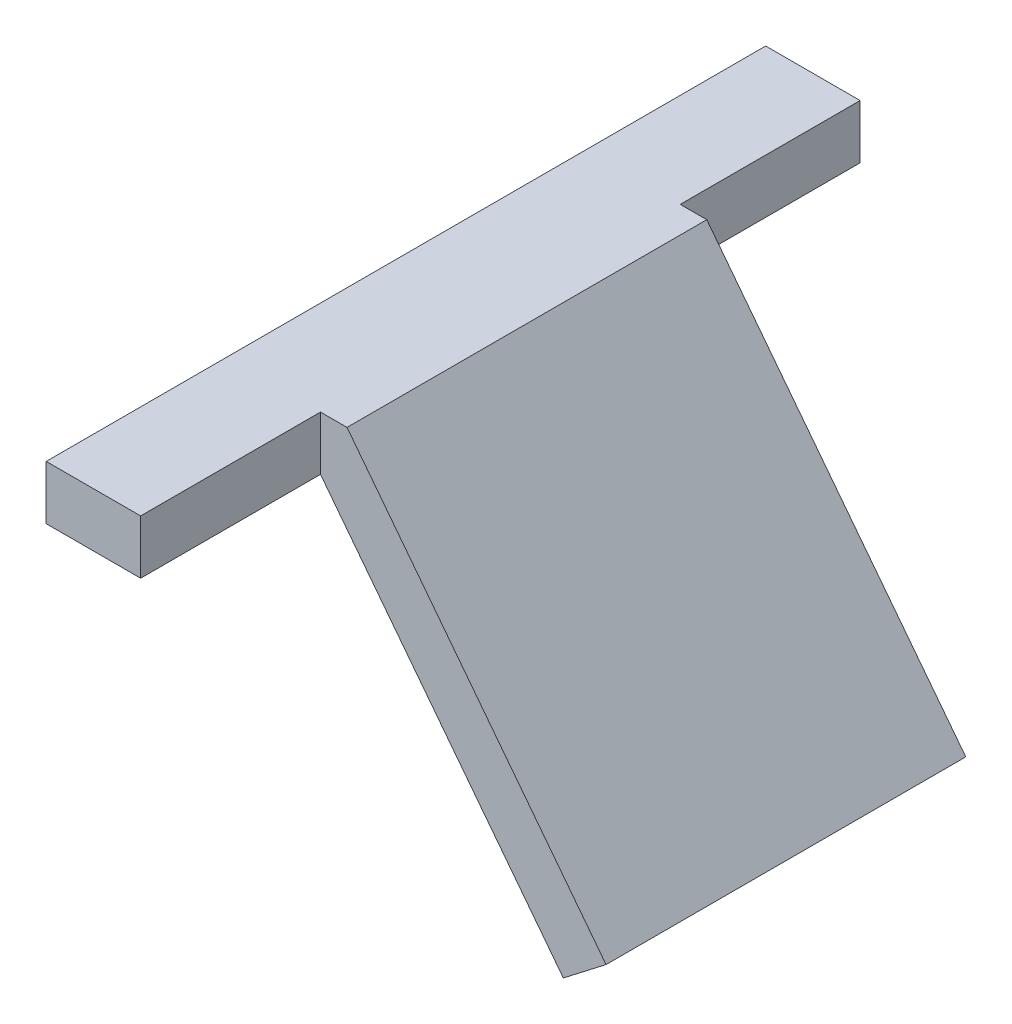
SolidWorks part; units mm, degrees
ref_plane "Front Plane" through (0, 0, 0) normal (0, 0, 1) x (1, 0, 0)
ref_plane "Top Plane" through (0, 0, 0) normal (0, 1, 0) x (1, 0, 0)
ref_plane "Right Plane" through (0, 0, 0) normal (1, 0, 0) x (0, 0, -1)
other "Configuration Table"
sketch "Sketch3" plane through (0, 0, 0) normal (0, 0, 1) x (1, 0, 0)
  line L0 (0, 0) -> (10.5, 0)
  line L1 (10.5, 0) -> (37.499, -34.9957)
  line L2 (0, 6) -> (13.4491, 6)
  line L3 (13.4491, 6) -> (42.2495, -31.3306)
  line L4 (0, 0) -> (0, 6)
  line L5 (37.499, -34.9957) -> (42.2495, -31.3306)
  dimension "D1" = 127.65
  dimension "D2" = 10.5
  dimension "D3" = 44.2
  dimension "D4" = 6
extrude "Boss-Extrude2" add sketch "Sketch3" along normal mid plane 40
sketch "Sketch4" plane through (0, 0, 20) normal (0, 0, 1) x (1, 0, 0)
  line L1 (0, 6) -> (10.5, 6)
  line L2 (0, 6) -> (0, 0)
  line L3 (0, 0) -> (10.5, 0)
  line L4 (10.5, 6) -> (10.5, 0)
extrude "Boss-Extrude3" add sketch "Sketch4" along normal blind 20
mirror "Mirror1" about plane through (0, 0, 0) normal (0, 0, 1) of "Boss-Extrude3"
